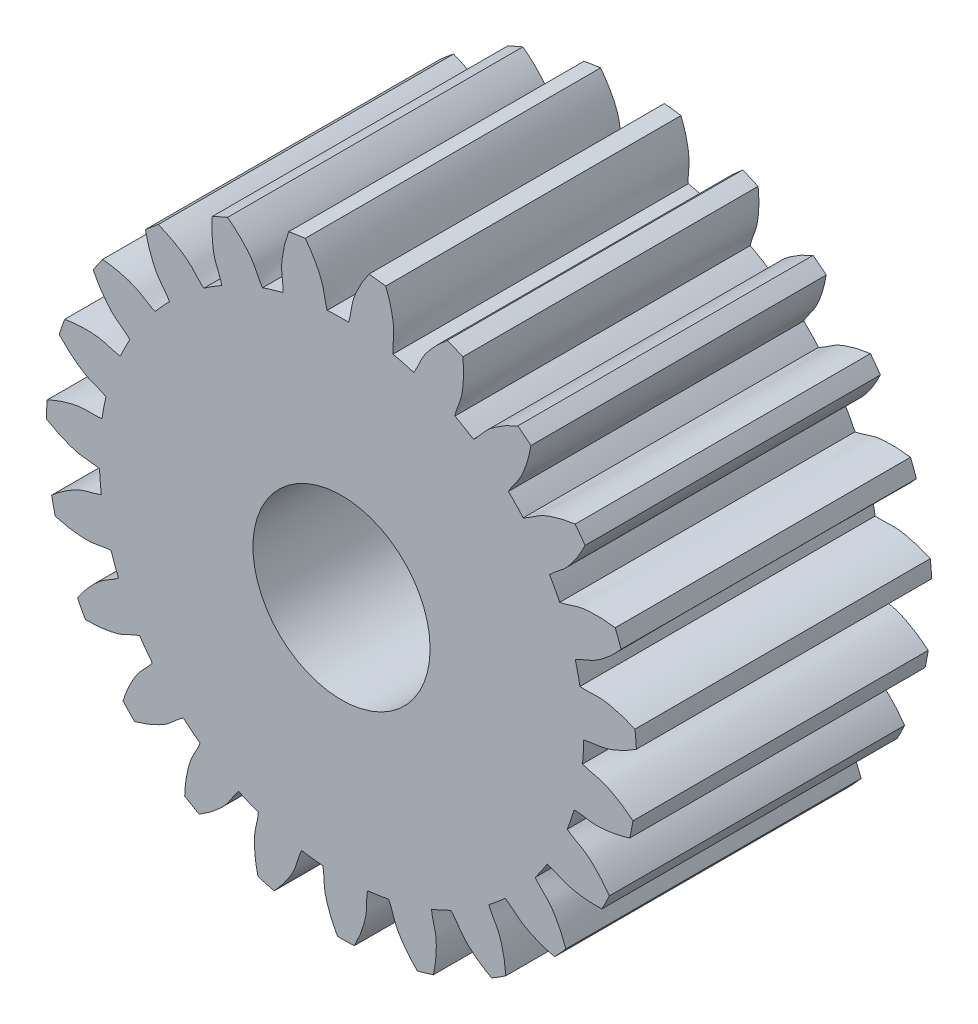
from build123d import *

# Parameters (mm, degrees)
SKETCH1_R           = 123
BOSS_EXTRUDE1_DEPTH = 150
BOSS_EXTRUDE2_DEPTH = 150
CIRPATTERN1_COUNT   = 23
CUT_EXTRUDE1_REACH  = 261.781
SKETCH5_R           = 45


with BuildPart() as part:
    # Sketch1 → Boss-Extrude1 (new body)
    with BuildSketch(Plane.XY):
        Circle(SKETCH1_R)
    extrude(amount=BOSS_EXTRUDE1_DEPTH)

    # Sketch2 → Boss-Extrude2 (add)
    with BuildSketch(Plane.XY):
        with BuildLine():
            ThreePointArc((149.066235202, 16.711000052), (149.481132956, 12.465588238), (149.775145906, 8.210095552))
            add(Edge.make_bspline(
                [(149.775145906, 8.210095552), (147.226230251, 6.542193143), (143.308555357, 4.272311714), (137.854181913, 1.950057985), (131.663374062, -0.156656217), (126.489917036, -0.141600789), (122.994762952, -1.135027005)],
                knots=[0, 0, 0, 0, 0.318898388, 0.471671526, 0.619977463, 1, 1, 1, 1], degree=3))
            ThreePointArc((122.994762952, -1.135027005), (122.574529024, 10.221782355), (121.107897063, 21.491330087))
            add(Edge.make_bspline(
                [(149.066235202, 16.711000052), (146.276266973, 17.933680199), (142.036737986, 19.523312939), (136.273061558, 20.91006673), (129.81882318, 21.962280364), (124.719318325, 21.090538141), (121.107897063, 21.491330087)],
                knots=[0, 0, 0, 0, 0.318898388, 0.471671526, 0.619977463, 1, 1, 1, 1], degree=3))
        make_face()
    boss_extrude2 = extrude(amount=BOSS_EXTRUDE2_DEPTH)

    # CirPattern1: Boss-Extrude2 ×23 about axis
    cirpattern1_axis = Axis((0, 0, 150), (0, 0, -1))
    for i in range(1, CIRPATTERN1_COUNT):
        add(boss_extrude2.rotate(cirpattern1_axis, i * 360 / CIRPATTERN1_COUNT))

    # Sketch5 → Cut-Extrude1 (cut, up to next)
    with BuildSketch(Plane.XY.offset(150), mode=Mode.PRIVATE) as cut_extrude1_sk1:
        Circle(SKETCH5_R)
    cut_extrude1_tool1 = extrude(cut_extrude1_sk1.sketch, amount=-CUT_EXTRUDE1_REACH, mode=Mode.PRIVATE) & part.part
    add(cut_extrude1_tool1.solids().sort_by_distance((0, 0, 150))[0], mode=Mode.SUBTRACT)


solid = part.part
